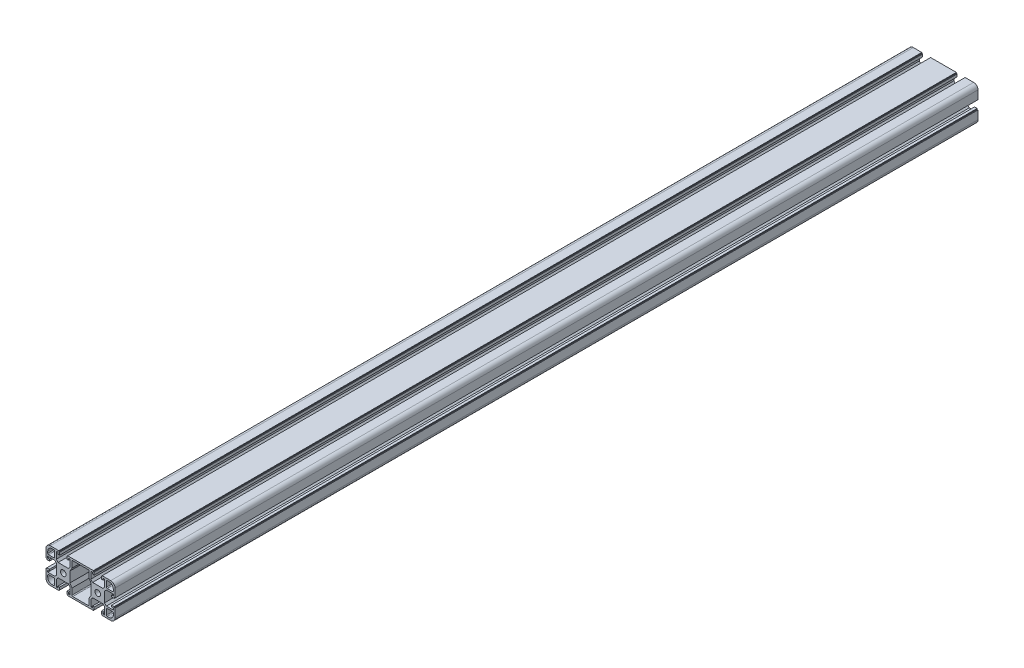
SolidWorks part; units mm, degrees
material "6061 合金"
ref_plane "前视基准面" through (0, 0, 0) normal (0, 0, 1) x (1, 0, 0)
ref_plane "上视基准面" through (0, 0, 0) normal (0, 1, 0) x (1, 0, 0)
ref_plane "右视基准面" through (0, 0, 0) normal (1, 0, 0) x (0, 0, -1)
sketch "草图1" plane through (0, 0, 0) normal (0, 0, 1) x (1, 0, 0)
  line L0 (0, 0) -> (0, 24.5989) construction
  line L1 (-5.1, 20) -> (-5.1, 19)
  line L2 (-20, 20) -> (-5.1, 20)
  line L3 (-20, 20) -> (-20, 5.1)
  line L4 (-20, -20) -> (-5.1, -20)
  line L5 (0, 0) -> (20, 0) construction
  line L6 (7.7, 6) -> (10, 10)
  line L7 (-5.1, 19) -> (-4.1, 19)
  line L8 (-4.1, 19) -> (-4.1, 16)
  line L9 (-4.1, 16) -> (-6.1, 16)
  line L10 (-6.1, 16) -> (-6.1, 18)
  line L11 (-6.1, 18) -> (-8, 18)
  line L12 (-8, 18) -> (-8, 10)
  line L13 (-8, 10) -> (-6, 7.7)
  line L14 (-6, 7.7) -> (6, 7.7)
  line L15 (8, 10) -> (6, 7.7)
  line L16 (8, 18) -> (8, 10)
  line L17 (6.1, 18) -> (8, 18)
  line L18 (6.1, 16) -> (6.1, 18)
  line L19 (4.1, 16) -> (6.1, 16)
  line L20 (4.1, 19) -> (4.1, 16)
  line L21 (5.1, 19) -> (4.1, 19)
  line L22 (5.1, 20) -> (5.1, 19)
  line L23 (5.1, -20) -> (5.1, -19)
  line L24 (5.1, -19) -> (4.1, -19)
  line L25 (4.1, -19) -> (4.1, -16)
  line L26 (4.1, -16) -> (6.1, -16)
  line L27 (6.1, -16) -> (6.1, -18)
  line L28 (6.1, -18) -> (8, -18)
  line L29 (8, -18) -> (8, -10)
  line L30 (8, -10) -> (6, -7.7)
  line L31 (-6, -7.7) -> (6, -7.7)
  line L32 (-8, -10) -> (-6, -7.7)
  line L33 (-8, -18) -> (-8, -10)
  line L34 (-6.1, -18) -> (-8, -18)
  line L35 (-6.1, -16) -> (-6.1, -18)
  line L36 (-4.1, -16) -> (-6.1, -16)
  line L37 (-4.1, -19) -> (-4.1, -16)
  line L38 (-5.1, -19) -> (-4.1, -19)
  line L39 (-5.1, -20) -> (-5.1, -19)
  line L40 (7.7, -6) -> (10, -10)
  line L41 (30, 10) -> (32.3, 6)
  line L42 (30, -10) -> (32.3, -6)
  line L55 (7.7, 6) -> (7.7, -6)
  line L57 (-19, -5.1) -> (-19, -4.1)
  line L58 (-7.7, 6) -> (-7.7, -6)
  line L59 (-10, 8) -> (-7.7, 6)
  line L60 (-18, 6.1) -> (-18, 8)
  line L61 (-19, 4.1) -> (-16, 4.1)
  line L62 (-16, 4.1) -> (-16, 6.1)
  line L63 (-20, 5.1) -> (-19, 5.1)
  line L64 (-18, -6.1) -> (-18, -8)
  line L65 (-16, -4.1) -> (-16, -6.1)
  line L66 (-16, -6.1) -> (-18, -6.1)
  line L67 (-16, 6.1) -> (-18, 6.1)
  line L68 (-10, -8) -> (-7.7, -6)
  line L69 (-19, 5.1) -> (-19, 4.1)
  line L70 (-18, -8) -> (-10, -8)
  line L71 (-18, 8) -> (-10, 8)
  line L72 (-20, -5.1) -> (-19, -5.1)
  line L73 (-19, -4.1) -> (-16, -4.1)
  line L74 (5.1, 20) -> (34.9, 20)
  line L75 (-20, -5.1) -> (-20, -20)
  line L76 (5.1, -20) -> (34.9, -20)
  line L78 (10, 18) -> (10, 10)
  line L79 (-18, 18) -> (-10, 18)
  line L80 (-18, 18) -> (-18, 10)
  line L81 (-18, 10) -> (-10, 10)
  line L82 (-10, 18) -> (-10, 10)
  line L85 (30, 18) -> (10, 18)
  line L89 (10, -18) -> (10, -10)
  line L90 (-10, -18) -> (-10, -10)
  line L91 (-18, -10) -> (-10, -10)
  line L92 (-18, -18) -> (-18, -10)
  line L93 (-18, -18) -> (-10, -18)
  line L94 (20, 0) -> (20, 30.8422) construction
  line L95 (58, -18) -> (50, -18)
  line L96 (58, -18) -> (58, -10)
  line L97 (58, -10) -> (50, -10)
  line L98 (50, -18) -> (50, -10)
  line L99 (30, -18) -> (30, -10)
  line L102 (10, -18) -> (30, -18)
  line L106 (50, 18) -> (50, 10)
  line L107 (58, 10) -> (50, 10)
  line L108 (58, 18) -> (58, 10)
  line L109 (58, 18) -> (50, 18)
  line L110 (30, 18) -> (30, 10)
  line L111 (60, -5.1) -> (60, -20)
  line L112 (59, -4.1) -> (56, -4.1)
  line L113 (60, -5.1) -> (59, -5.1)
  line L114 (58, 8) -> (50, 8)
  line L115 (58, -8) -> (50, -8)
  line L116 (59, 5.1) -> (59, 4.1)
  line L117 (50, -8) -> (47.7, -6)
  line L118 (56, 6.1) -> (58, 6.1)
  line L119 (56, -6.1) -> (58, -6.1)
  line L120 (56, -4.1) -> (56, -6.1)
  line L121 (58, -6.1) -> (58, -8)
  line L122 (60, 5.1) -> (59, 5.1)
  line L123 (56, 4.1) -> (56, 6.1)
  line L124 (59, 4.1) -> (56, 4.1)
  line L125 (58, 6.1) -> (58, 8)
  line L126 (50, 8) -> (47.7, 6)
  line L127 (47.7, 6) -> (47.7, -6)
  line L128 (59, -5.1) -> (59, -4.1)
  line L130 (32.3, 6) -> (32.3, -6)
  line L144 (45.1, -20) -> (45.1, -19)
  line L145 (45.1, -19) -> (44.1, -19)
  line L146 (44.1, -19) -> (44.1, -16)
  line L147 (44.1, -16) -> (46.1, -16)
  line L148 (46.1, -16) -> (46.1, -18)
  line L149 (46.1, -18) -> (48, -18)
  line L150 (48, -18) -> (48, -10)
  line L151 (48, -10) -> (46, -7.7)
  line L152 (46, -7.7) -> (34, -7.7)
  line L153 (32, -10) -> (34, -7.7)
  line L154 (32, -18) -> (32, -10)
  line L155 (33.9, -18) -> (32, -18)
  line L156 (33.9, -16) -> (33.9, -18)
  line L157 (35.9, -16) -> (33.9, -16)
  line L158 (35.9, -19) -> (35.9, -16)
  line L159 (34.9, -19) -> (35.9, -19)
  line L160 (34.9, -20) -> (34.9, -19)
  line L161 (34.9, 20) -> (34.9, 19)
  line L162 (34.9, 19) -> (35.9, 19)
  line L163 (35.9, 19) -> (35.9, 16)
  line L164 (35.9, 16) -> (33.9, 16)
  line L165 (33.9, 16) -> (33.9, 18)
  line L166 (33.9, 18) -> (32, 18)
  line L167 (32, 18) -> (32, 10)
  line L168 (32, 10) -> (34, 7.7)
  line L169 (46, 7.7) -> (34, 7.7)
  line L170 (48, 10) -> (46, 7.7)
  line L171 (48, 18) -> (48, 10)
  line L172 (46.1, 18) -> (48, 18)
  line L173 (46.1, 16) -> (46.1, 18)
  line L174 (44.1, 16) -> (46.1, 16)
  line L175 (44.1, 19) -> (44.1, 16)
  line L176 (45.1, 19) -> (44.1, 19)
  line L177 (60, -20) -> (45.1, -20)
  line L178 (60, 20) -> (60, 5.1)
  line L179 (60, 20) -> (45.1, 20)
  line L180 (45.1, 20) -> (45.1, 19)
  circle A0 centre (0, 0) radius 3.25
  circle A1 centre (40, 0) radius 3.25
  point P19 (0, 7.7)
  point P27 (0, -7.7)
  point P102 (40, -7.7)
  point P103 (40, 7.7)
  dimension "D12" = 10
  dimension "D23" = 6.5
  dimension "D2" = 40
  dimension "D3" = 8.2
  dimension "D4" = 10.2
  dimension "D5" = 1
  dimension "D6" = 2
  dimension "D7" = 4
  dimension "D8" = 2
  dimension "D9" = 16
  dimension "D10" = 12.3
  dimension "D11" = 12
  dimension "D13" = 20
  dimension "D14" = 80
  dimension "D15" = 2
  dimension "D16" = 10
  dimension "D17" = 8.2
  dimension "D18" = 10.2
  dimension "D19" = 12.2
  dimension "D20" = 1
  dimension "D21" = 4
  dimension "D22" = 12
  dimension "D24" = 2
  dimension "D25" = 2
  dimension "D26" = 12.3
  dimension "D27" = 10
extrude "拉伸1" add sketch "草图1" along normal blind 1000
fillet "圆角1" radius 5 8 edges at (-20, -20, 500) (-20, 20, 500) (-18, -18, 500) (-18, 18, 500) (60, -20, 500) (60, 20, 500) (58, -18, 500) (58, 18, 500)
fillet "圆角2" radius 1 16 edges at (-10, -10, 500) (-18, -10, 500) (-10, 18, 500) (10, 18, 500) (-10, -18, 500) (-10, 10, 500) (-18, 10, 500) (50, 18, 500) (50, 10, 500) (58, 10, 500) (58, -10, 500) (50, -10, 500) (50, -18, 500) (30, 18, 500) (30, -18, 500) (10, -18, 500)
